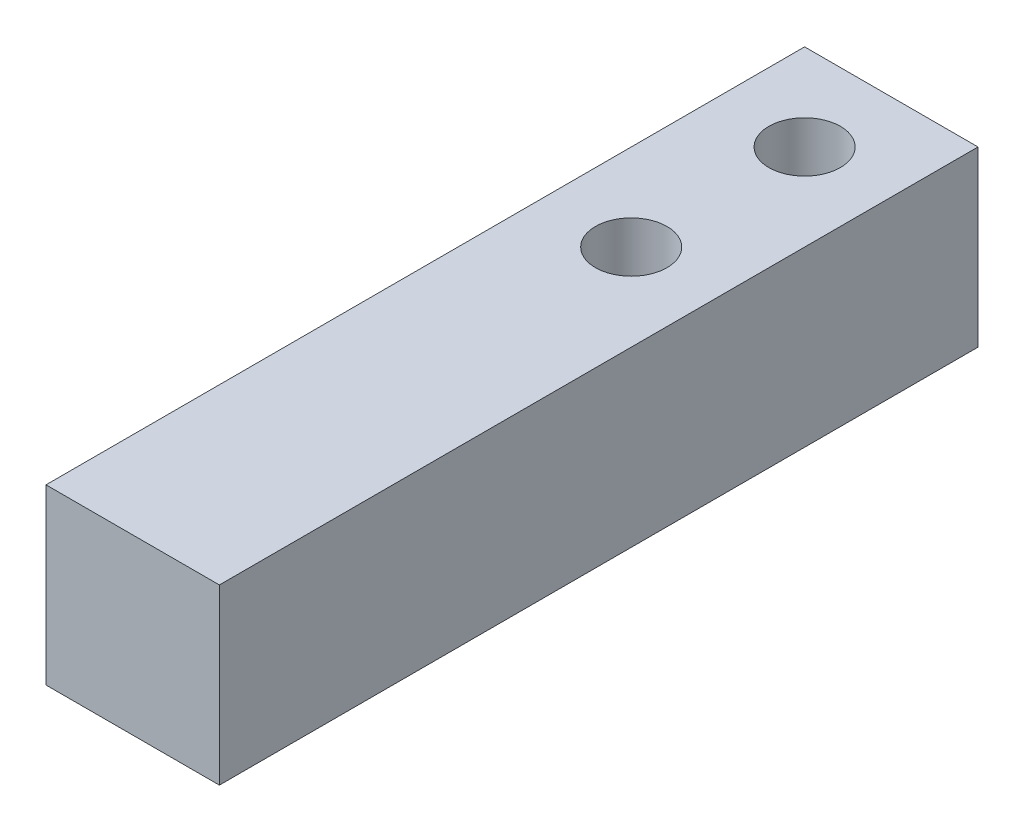
from build123d import *

# Parameters (mm, degrees)
SKETCH_1_W         = 8
SKETCH_1_H         = 8
EXTRUDE_1_DEPTH    = 35
HOLE_WIZARD_M4_1_D = 3.3


with BuildPart() as part:
    # 草图1 → 凸台-拉伸1 (new body)
    with BuildSketch(Plane.XY):
        Rectangle(SKETCH_1_W, SKETCH_1_H)
    extrude(amount=EXTRUDE_1_DEPTH)

    # M4 螺纹孔1 (through all)
    with Locations(Plane(origin=(0, -4, 0), x_dir=(-1, 0, 0), z_dir=(0, -1, 0))):
        with Locations((0, -12), (0, -4)):
            Hole(HOLE_WIZARD_M4_1_D / 2)


solid = part.part
